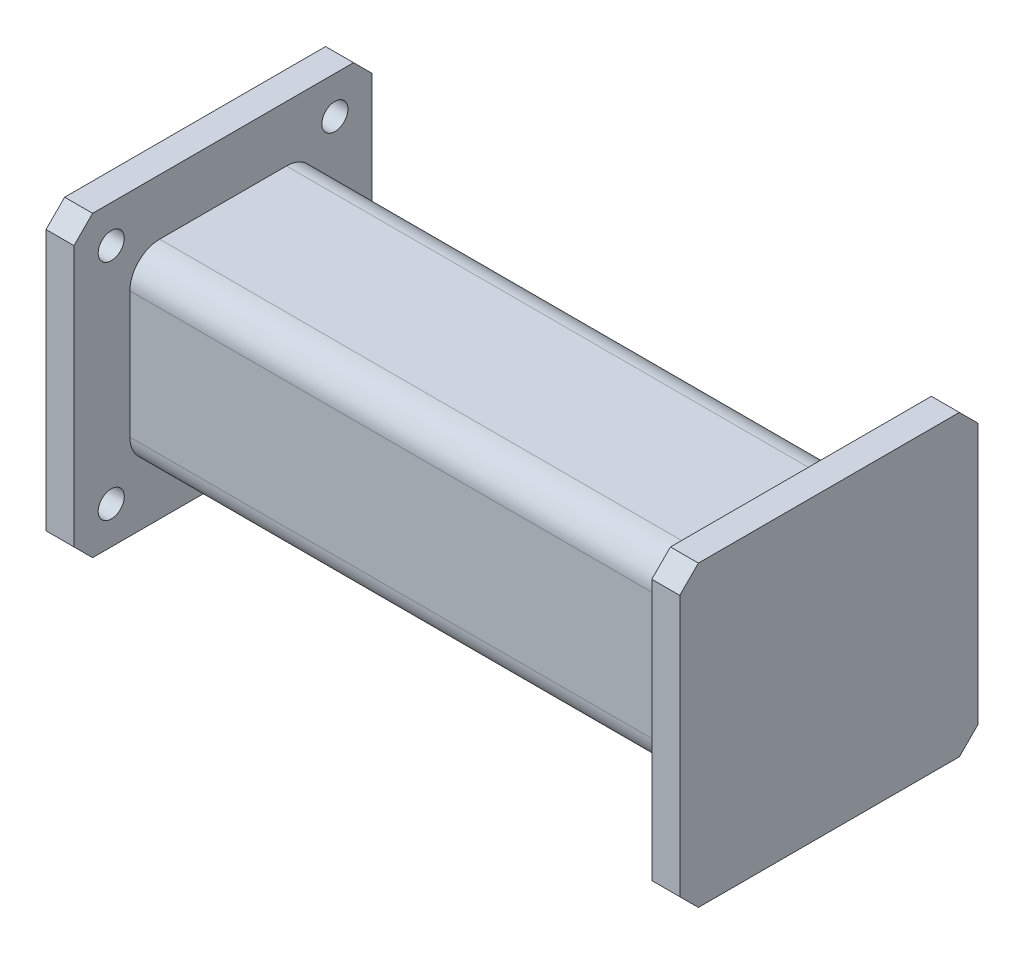
from build123d import *

# Parameters (mm, degrees)
BOSS_EXTRUDE1_DEPTH            = 15
BOSS_EXTRUDE2_DEPTH            = 310
F_14_0_14_DIAMETER_HOLE1_D     = 14
F_14_0_14_DIAMETER_HOLE1_DEPTH = 15


with BuildPart() as part:
    # Sketch1 → Boss-Extrude1 (new body)
    with BuildSketch(Plane(origin=(0, 0, 0), x_dir=(0, 0, -1), z_dir=(1, 0, 0))):
        Polygon((0, 150), (10, 160), (150, 160), (160, 150), (160, 10), (150, 0), (10, 0), (0, 10), align=None)
    boss_extrude1 = extrude(amount=BOSS_EXTRUDE1_DEPTH)

    # Sketch2 → Boss-Extrude2 (add)
    with BuildSketch(Plane(origin=(15, 0, 0), x_dir=(0, 0, -1), z_dir=(1, 0, 0))):
        with BuildLine():
            Line((46, 130), (114, 130))
            ThreePointArc((114, 130), (125.313708499, 125.313708499), (130, 114))
            Line((130, 114), (130, 46))
            ThreePointArc((130, 46), (125.313708499, 34.686291501), (114, 30))
            Line((114, 30), (46, 30))
            ThreePointArc((46, 30), (34.686291501, 34.686291501), (30, 46))
            Line((30, 46), (30, 114))
            ThreePointArc((30, 114), (34.686291501, 125.313708499), (46, 130))
        make_face()
        with BuildLine():
            Line((46, 122), (114, 122))
            ThreePointArc((114, 122), (119.656854249, 119.656854249), (122, 114))
            Line((122, 114), (122, 46))
            ThreePointArc((122, 46), (119.656854249, 40.343145751), (114, 38))
            Line((114, 38), (46, 38))
            ThreePointArc((46, 38), (40.343145751, 40.343145751), (38, 46))
            Line((38, 46), (38, 114))
            ThreePointArc((38, 114), (40.343145751, 119.656854249), (46, 122))
        make_face(mode=Mode.SUBTRACT)
    extrude(amount=BOSS_EXTRUDE2_DEPTH)

    # Mirror1: Boss-Extrude1 across plane
    add(boss_extrude1.mirror(Plane(origin=(170, 0, 0), x_dir=(0, 0, 1), z_dir=(1, 0, 0))))

    # Ø14.0 (14) Diameter Hole1
    with Locations(Plane(origin=(15, 140, -140), x_dir=(0, 0, 1), z_dir=(1, 0, 0))):
        with Locations((0, 0), (0, 120), (120, 0), (120, 120)):
            Hole(F_14_0_14_DIAMETER_HOLE1_D / 2, depth=F_14_0_14_DIAMETER_HOLE1_DEPTH)


solid = part.part
